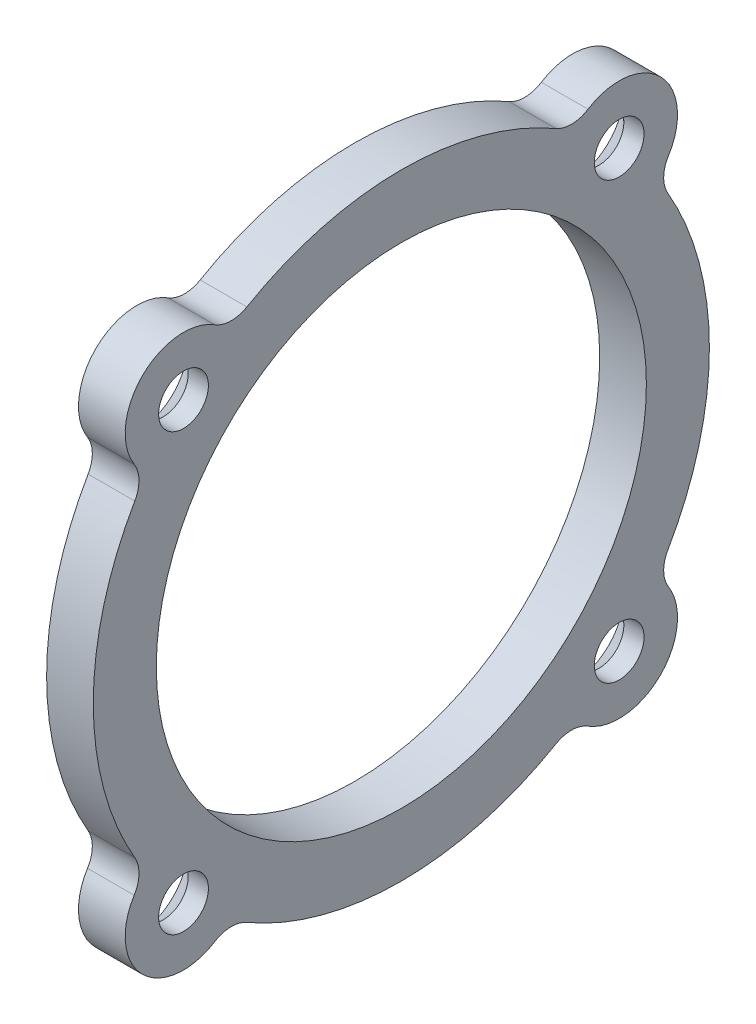
from build123d import *

# Parameters (mm, degrees)
SKETCH_1_R               = 15.75
SKETCH_1_R_2             = 1.6
EXTRUDE_1_DEPTH          = 3
PATTERN_CIRCULAR_1_COUNT = 4
FILLET_1_R               = 2


with BuildPart() as part:
    # 草图1 → 凸台-拉伸1 (new body)
    with BuildSketch(Plane(origin=(0, 0, 0), x_dir=(0, 0, -1), z_dir=(1, 0, 0))):
        with BuildLine():
            ThreePointArc((-16.389345303, 11.109876711), (-19.8, 0), (-16.389345303, -11.109876711))
            ThreePointArc((-16.389345303, -11.109876711), (-16.652364697, -16.652364697), (-11.109876711, -16.389345303))
            ThreePointArc((-11.109876711, -16.389345303), (0, -19.8), (11.109876711, -16.389345303))
            ThreePointArc((11.109876711, -16.389345303), (16.652364697, -16.652364697), (16.389345303, -11.109876711))
            ThreePointArc((16.389345303, -11.109876711), (19.8, 0), (16.389345303, 11.109876711))
            ThreePointArc((16.389345303, 11.109876711), (16.652364697, 16.652364697), (11.109876711, 16.389345303))
            ThreePointArc((11.109876711, 16.389345303), (0, 19.8), (-11.109876711, 16.389345303))
            ThreePointArc((-11.109876711, 16.389345303), (-16.652364697, 16.652364697), (-16.389345303, 11.109876711))
        make_face()
        Circle(SKETCH_1_R, mode=Mode.SUBTRACT)
        with Locations((14.000714267, -14.000714267)):
            Circle(SKETCH_1_R_2, mode=Mode.SUBTRACT)
        with Locations((-14.000714267, -14.000714267)):
            Circle(SKETCH_1_R_2, mode=Mode.SUBTRACT)
        with Locations((-14.000714267, 14.000714267)):
            Circle(SKETCH_1_R_2, mode=Mode.SUBTRACT)
        with Locations((14.000714267, 14.000714267)):
            Circle(SKETCH_1_R_2, mode=Mode.SUBTRACT)
    extrude(amount=EXTRUDE_1_DEPTH)

    # 草图2 → 切除-旋转1 (revolve, cut)
    with BuildSketch(Plane(origin=(0, 0, 0), x_dir=(1, 0, 0), z_dir=(0, -0.7071067811865581, 0.707106781186537)), mode=Mode.PRIVATE) as cut_revolve_1_sk:
        Polygon((0, 19.8), (0, 23.1), (3.3, 19.8), align=None)
    cut_revolve_1 = revolve(cut_revolve_1_sk.sketch.rotate(Axis((3.3, 14.000714267, 14.000714267), (-1, 0, 0)), 315), axis=Axis((3.3, 14.000714267, 14.000714267), (-1, 0, 0)), mode=Mode.SUBTRACT)

    # 阵列(圆周)1: 切除-旋转1 ×4 about axis
    pattern_circular_1_axis = Axis((0, 0, 0), (1, 0, 0))
    for i in range(1, PATTERN_CIRCULAR_1_COUNT):
        add(cut_revolve_1.rotate(pattern_circular_1_axis, i * 360 / PATTERN_CIRCULAR_1_COUNT), mode=Mode.SUBTRACT)

    # 圆角1
    fillet_1_edges = [part.edges().sort_by_distance(p)[0] for p in [
        (1.5, -11.109876711, -16.389345303),
        (1.5, -16.389345303, -11.109876711),
        (1.5, -16.389345303, 11.109876711),
        (1.5, -11.109876711, 16.389345303),
        (1.5, 11.109876711, 16.389345303),
        (1.5, 16.389345303, 11.109876711),
        (1.5, 16.389345303, -11.109876711),
        (1.5, 11.109876711, -16.389345303),
    ]]
    fillet(fillet_1_edges, radius=FILLET_1_R)


solid = part.part
